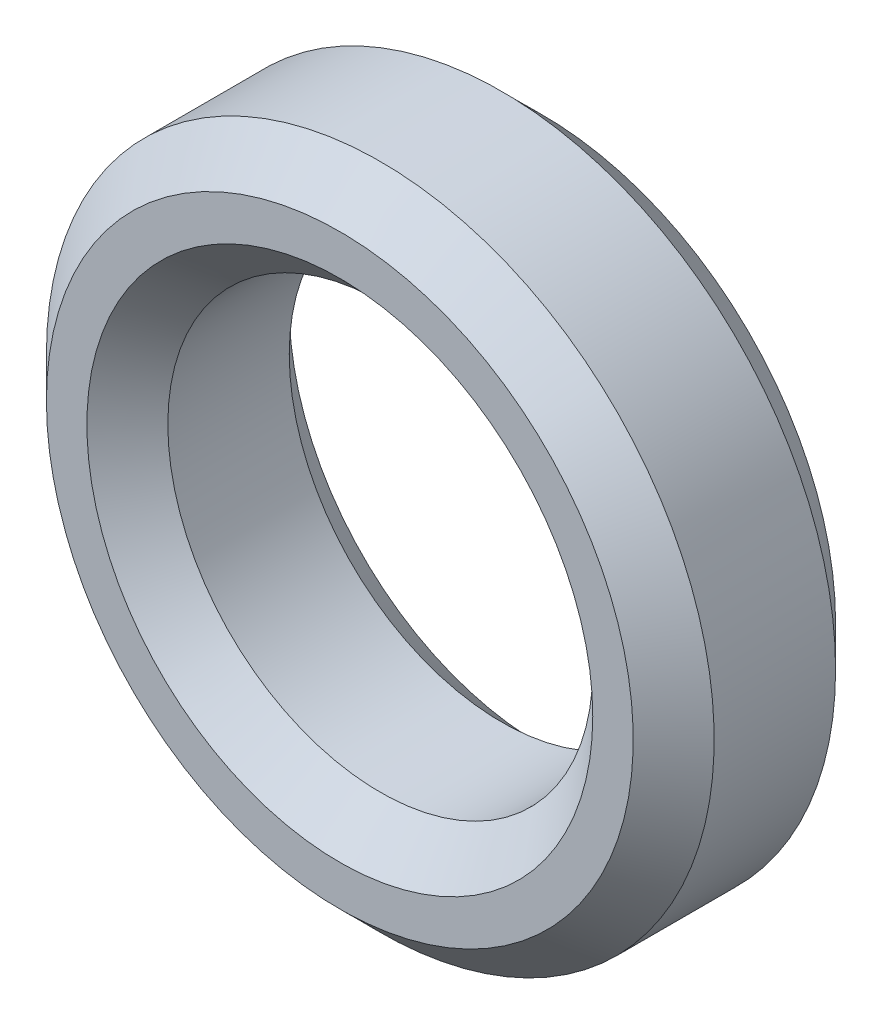
from build123d import *

# Parameters (mm, degrees)
SKETCH1_R           = 1.65
SKETCH1_R_2         = 1.05
BOSS_EXTRUDE1_DEPTH = 1
CHAMFER1_SIZE       = 0.2


with BuildPart() as part:
    # Sketch1 → Boss-Extrude1 (new body)
    with BuildSketch(Plane.XY):
        Circle(SKETCH1_R)
        Circle(SKETCH1_R_2, mode=Mode.SUBTRACT)
    extrude(amount=BOSS_EXTRUDE1_DEPTH)

    # Chamfer1
    chamfer1_edges = [part.edges().sort_by_distance(p)[0] for p in [
        (-1.65, 0, 0),
        (-1.65, 0, 1),
        (-1.05, 0, 0),
        (-1.05, 0, 1),
    ]]
    chamfer(chamfer1_edges, length=CHAMFER1_SIZE)


solid = part.part
